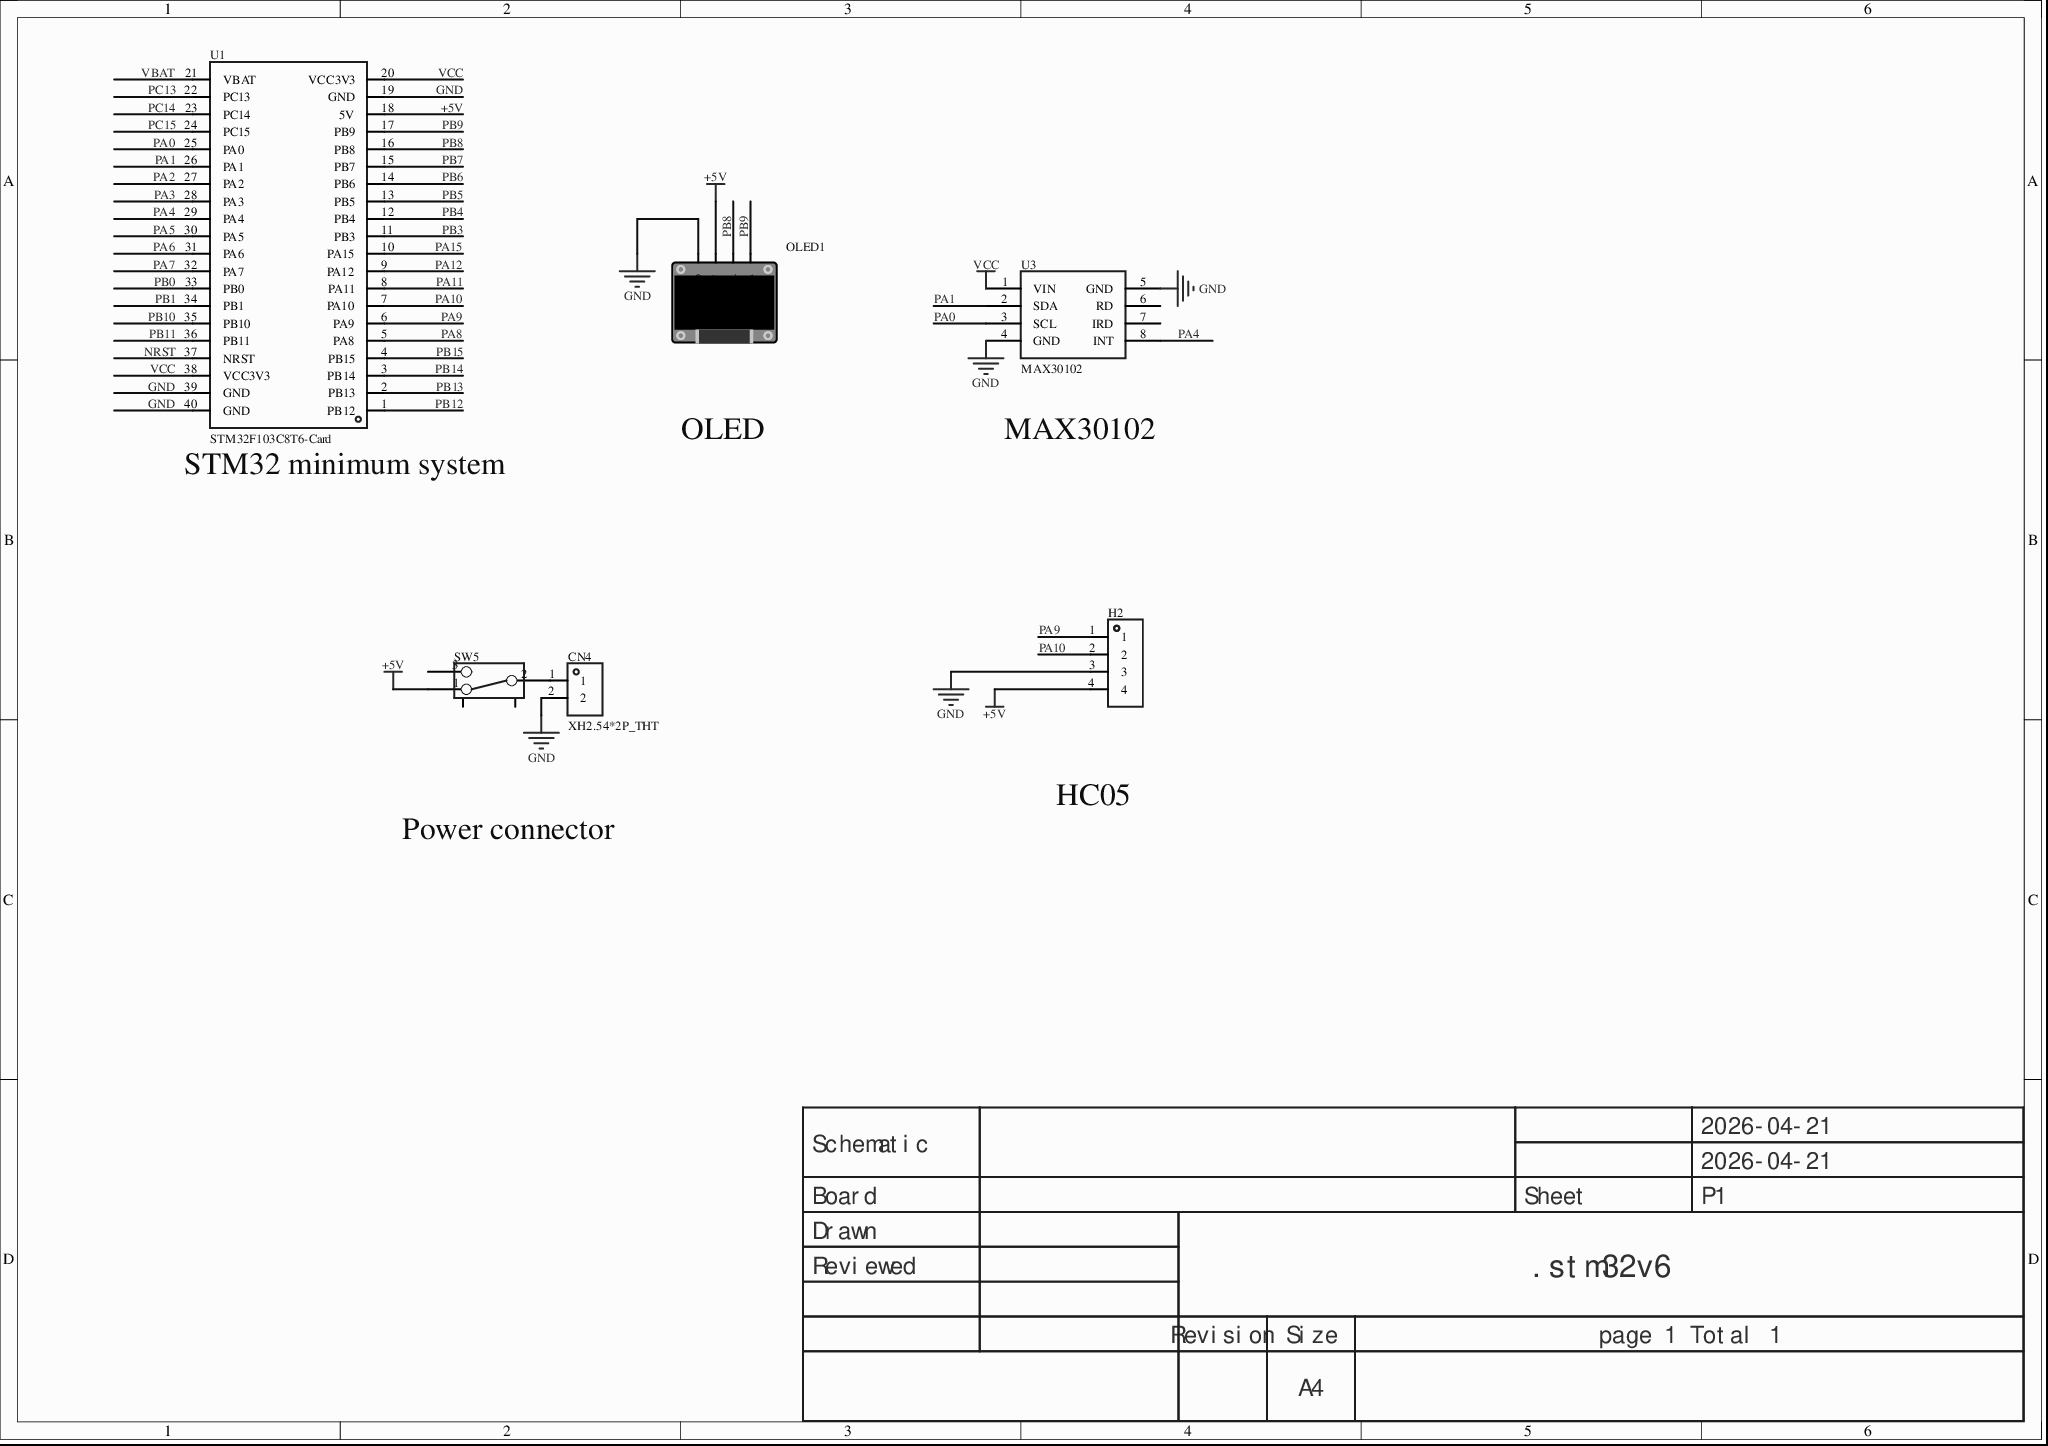
[diagram p0: MISC50728-3.schdoc]
# Altium project MISC50728-2.PrjPcb
1 sheet, 6 parts. Net scope: global (net labels, ports and power ports of the same name join across sheets).
Board file: MISC50728.pcbdoc

## Sheet MISC50728-3.schdoc
size 297 x 209 mm; Version: V1.0; @Project Name: MISC50728; @Page Count: 1; @Update Date: 2026-04-21; @Create Date: 2026-04-21; @Schematic Name: MISC50728; @Page No: 1; @Create Time: 23:22:16; @Update Time: 17:32:40; @Board Name: MISC50728

### Parts
CN4  XH2.54*2P_THT  [CONN-TH_2P-P2.50-XH2.54-2P]
H2  (no value)  [HDR-TH_4P-P2.54-V-F]
OLED1  (no value)  [0.96OLED_4P]
SW5  (no value)  [拨动开关]
U1  STM32F103C8T6-Card  [CONN-TH_L53.3-W22.9_STM32F103C8T6-CARD]
U3  MAX30102  [MAX30102]

### Nets
+5V: H2.4 OLED1.2(VCC) SW5.1 U1.18(5V)
GND: CN4.2 H2.3 OLED1.1(GND) U1.19(GND) U1.39(GND) U1.40(GND) U3.4(GND) U3.5(GND)
VCC: U1.20(VCC3V3) U1.38(VCC3V3) U3.1(VIN)
NRST: U1.37(NRST)
PA0: U1.25(PA0) U3.3(SCL)
PA1: U1.26(PA1) U3.2(SDA)
PA2: U1.27(PA2)
PA3: U1.28(PA3)
PA4: U1.29(PA4) U3.8(INT)
PA5: U1.30(PA5)
PA6: U1.31(PA6)
PA7: U1.32(PA7)
PA8: U1.5(PA8)
PA9: H2.1 U1.6(PA9)
PA10: H2.2 U1.7(PA10)
PA11: U1.8(PA11)
PA12: U1.9(PA12)
PA15: U1.10(PA15)
PB0: U1.33(PB0)
PB1: U1.34(PB1)
PB3: U1.11(PB3)
PB4: U1.12(PB4)
PB5: U1.13(PB5)
PB6: U1.14(PB6)
PB7: U1.15(PB7)
PB8: OLED1.3(SCL) U1.16(PB8)
PB9: OLED1.4(SDA) U1.17(PB9)
PB10: U1.35(PB10)
PB11: U1.36(PB11)
PB12: U1.1(PB12)
PB13: U1.2(PB13)
PB14: U1.3(PB14)
PB15: U1.4(PB15)
PC13: U1.22(PC13)
PC14: U1.23(PC14)
PC15: U1.24(PC15)
VBAT: U1.21(VBAT)
NetCN4_1: CN4.1 SW5.2

Not connected (* = marked no-connect by the designer): SW5 3 4 5; U3 6(RD) 7(IRD)

### Notes on the sheet
- (near U1) STM32 minimum system
- OLED
- MAX30102
- 核心控制单元：STM32F103C8T6最小系统板
  0.96英寸OLED显示屏：SCL=PB8,SDA=PB9
  MAX30102:SCL=PA0,SDA=PA1,INT=PA4
  HC-05:TX=PA10,RX=PA9
  增加一个电源供电，放一节5v锂电池
  增加一个电源开关
  STM32F103C8T6最小系统板
- Power connector
- HC05
- Labels drawn without touching a wire or pin: VCC
- 2026-04-21
- Schematic
- Board
- Sheet
- P1
- Drawn
- Reviewed
- .stm32v6
- Revision
- Size
- A4
- page 1 Total 1

### Library data of the parts
CN4 = XH2.54*2P_直插: 3D Model: 325c595e30db4df8abe76612dd40b0fa0819f05c4eef4c71ace90d822a990e87; 3D Model Transform: 295.275,228.346,0,180,0,0,-0.002,-20.079,-137.795; AddInBom: yes; Symbol: XH2.54*2P_THT; Device: XH2.54*2P_THT; LCSC Part Name: XH2.54*2P_直插; Supplier Part: C9900008615; Manufacturer Part: XH2.54*2P_直插; Supplier Footprint: XH2.54_2P; JLCPCB Part Class: Extended Part; Supplier: LCSC; ConvertToPcb: yes; FootprintName: CONN-TH_2P-P2.50-XH2.54-2P; ModelName: CONN-TH_2P-P2.50-XH2.54-2P
H2 = HDR-F_2.54_1x4P: Symbol: 2.54-1*4P female; 3D Model: d187812051054f85879fcaa51a310d8e0819f05c4eef4c71ace90d822a990e87; 3D Model Transform: 419.6842,98.464,0,0,0,0,0,0,-118.11; ConvertToPcb: yes; Device: HDR-F_2.54_1x4P; Supplier Part: C2718488; Supplier Footprint: 插件; FootprintName: HDR-TH_4P-P2.54-V-F; AddInBom: yes; ModelName: HDR-TH_4P-P2.54-V-F
OLED1 = 0.96OLED模块_4P: Symbol: 0.96OLED module_4P; ConvertToPcb: yes; ModelId: 79c000fdb68d45a296c2e9bedf4f9055; ModelTransform: 1393.69792,1318.895,0,0,0,0,0,-560.079,-137.795; Device: 0.96OLED module_4P; AddInBom: yes; FootprintName: 0.96OLED_4P; Supplier Footprint: 插件; ModelName: 0.96OLED_4P
SW5 = 拨动开关_正: Symbol: Toggle switch; Device: Toggle switch_pos; ConvertToPcb: yes; ModelId: 4321fe59a4074cbfb4989553f297c68f0819f05c4eef4c71ace90d822a990e87; ModelName: SW-TH_SS-12D02-VG4; ModelTransform: 370.09,208.7,472.35,0,0,0,0,0,-110; AddInBom: yes; Supplier Footprint: 插件; FootprintName: Toggle switch
U1 = STM32F103C8T6-Card: AddInBom: yes; Symbol: STM32F103C8T6-CARD; Device: STM32F103C8T6-Card; LCSC Part Name: STM32F103C8T6-Card; SupplierPart: C9900077949; ManufacturerPart: STM32F103C8T6-Card; Supplier Footprint: 插件; Supplier: LCSC; ConvertToPcb: yes; FootprintName: CONN-TH_L53.3-W22.9_STM32F103C8T6-CARD
U3 = MAX30102: AddInBom: yes; Symbol: MAX30102; Device: MAX30102; ConvertToPcb: yes; FootprintName: MAX30102